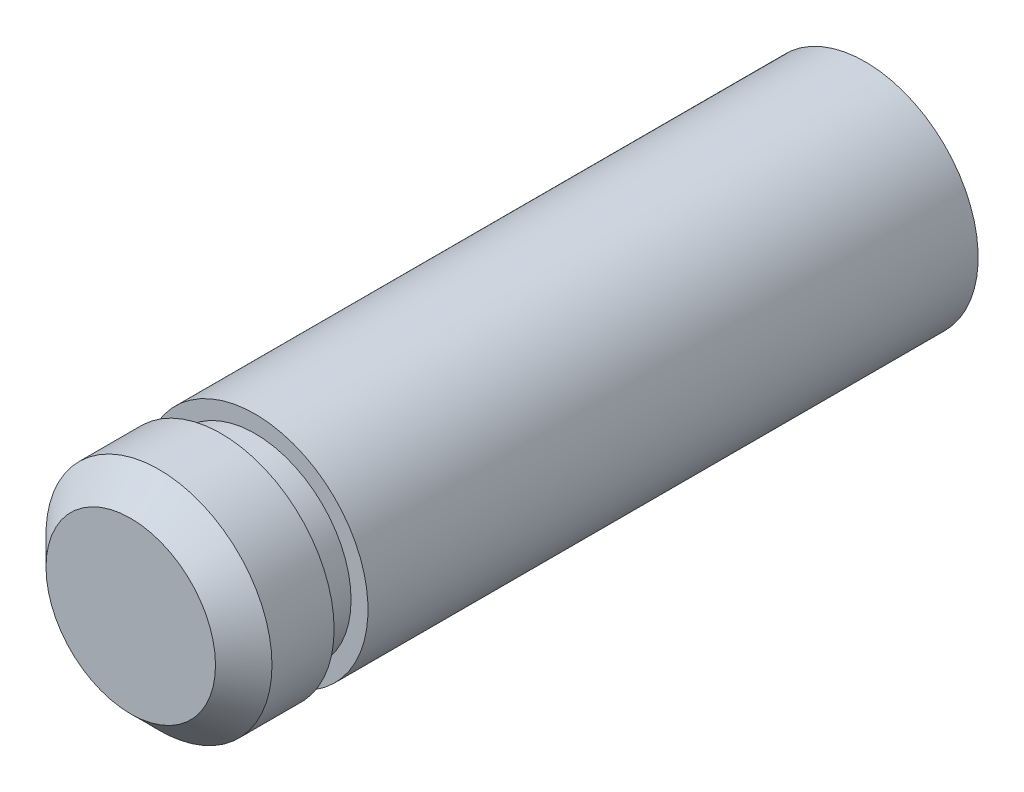
from build123d import *

# Parameters (mm, degrees)
SKETCH1_R           = 2
BOSS_EXTRUDE1_DEPTH = 10.8
SKETCH2_R           = 1.7
BOSS_EXTRUDE2_DEPTH = 0.6
SKETCH3_R           = 2
BOSS_EXTRUDE3_DEPTH = 1.6
CHAMFER1_SIZE       = 0.5


with BuildPart() as part:
    # Sketch1 → Boss-Extrude1 (new body)
    with BuildSketch(Plane.XY):
        with Locations(Location((0, 0, 0), (0, 0, 180))):
            Circle(SKETCH1_R)
    extrude(amount=BOSS_EXTRUDE1_DEPTH)

    # Sketch2 → Boss-Extrude2 (add)
    with BuildSketch(Plane.XY.offset(10.8)):
        Circle(SKETCH2_R)
    extrude(amount=BOSS_EXTRUDE2_DEPTH)

    # Sketch3 → Boss-Extrude3 (add)
    with BuildSketch(Plane.XY.offset(11.4)):
        with Locations(Location((0, 0, 0), (0, 0, 180))):
            Circle(SKETCH3_R)
    extrude(amount=BOSS_EXTRUDE3_DEPTH)

    # Chamfer1
    chamfer1_edges = [part.edges().sort_by_distance(p)[0] for p in [
        (2, 0, 13),
    ]]
    chamfer(chamfer1_edges, length=CHAMFER1_SIZE)


solid = part.part
